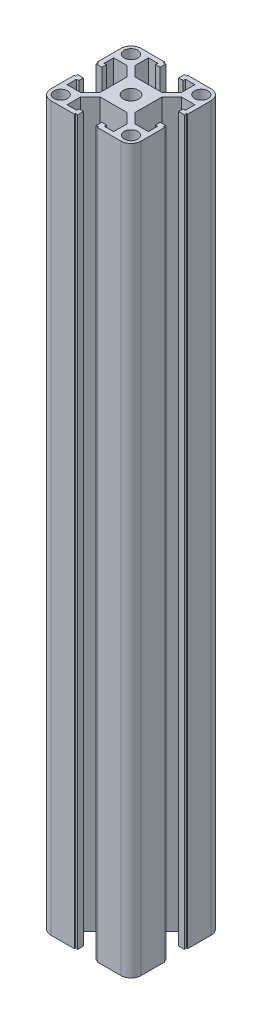
SolidWorks part; units mm, degrees
ref_plane "主视基准图" through (0, 0, 0) normal (0, 0, 1) x (1, 0, 0)
ref_plane "上视基准图" through (0, 0, 0) normal (0, 1, 0) x (1, 0, 0)
ref_plane "右视基准图" through (0, 0, 0) normal (1, 0, 0) x (0, 0, -1)
sketch "草图1" plane through (0, 0, 0) normal (0, 0, 1) x (1, 0, 0)
  line L0 (0, 0) -> (0, 320)
  dimension "D1" = 320
other "结构构件1"
ref_plane "基准面1" through (0, 0, 0) normal (0, 1, 0) x (-1, 0, 0)
sketch "Sketch16" plane through (0, 0, 0) normal (0, 1, 0) x (-1, 0, 0)
  line L0 (-5.1, 20) -> (-5.1, 19.5)
  line L1 (-5.1, 19.5) -> (-4.1, 19.5)
  line L2 (-4.1, 19.5) -> (-4.1, 17)
  line L3 (-6.1, 18) -> (-10.3, 18)
  line L4 (-15.5, -20) -> (-5.1, -20)
  line L5 (-20, -15.5) -> (-20, -5.1)
  line L6 (15.5, 20) -> (5.1, 20)
  line L7 (20, 15.5) -> (20, 5.1)
  line L8 (0, 14.8756) -> (0, 0) construction
  line L9 (0, 0) -> (14.1675, 0) construction
  line L10 (-10.3, 18) -> (-10.3, 12)
  line L11 (-10.3, 12) -> (-6, 7.7)
  line L12 (-6, 7.7) -> (6, 7.7)
  line L13 (10.3, 12) -> (6, 7.7)
  line L14 (10.3, 18) -> (10.3, 12)
  line L15 (6.1, 18) -> (10.3, 18)
  line L16 (4.1, 19.5) -> (4.1, 17)
  line L17 (5.1, 19.5) -> (4.1, 19.5)
  line L18 (5.1, 20) -> (5.1, 19.5)
  line L19 (-5.1, 20) -> (-15.5, 20)
  line L20 (20, 5.1) -> (19.5, 5.1)
  line L21 (0, 0) -> (-15.5563, 15.5563) construction
  line L22 (0, 0) -> (-15.5563, -15.5563) construction
  line L25 (19.5, 5.1) -> (19.5, 4.1)
  line L26 (19.5, 4.1) -> (17, 4.1)
  line L27 (17, 6.1) -> (17, 4.1)
  line L28 (18, 6.1) -> (17, 6.1)
  line L29 (18, 6.1) -> (18, 10.3)
  line L30 (18, 10.3) -> (12, 10.3)
  line L31 (12, 10.3) -> (7.7, 6)
  line L32 (7.7, 6) -> (7.7, -6)
  line L33 (12, -10.3) -> (7.7, -6)
  line L34 (18, -10.3) -> (12, -10.3)
  line L35 (18, -6.1) -> (18, -10.3)
  line L36 (18, -6.1) -> (17, -6.1)
  line L37 (17, -4.1) -> (17, -6.1)
  line L38 (19.5, -4.1) -> (17, -4.1)
  line L39 (19.5, -5.1) -> (19.5, -4.1)
  line L40 (20, -5.1) -> (19.5, -5.1)
  line L41 (5.1, -20) -> (5.1, -19.5)
  line L42 (5.1, -19.5) -> (4.1, -19.5)
  line L43 (4.1, -19.5) -> (4.1, -17)
  line L44 (6.1, -17) -> (4.1, -17)
  line L45 (6.1, -18) -> (6.1, -17)
  line L46 (6.1, -18) -> (10.3, -18)
  line L47 (10.3, -18) -> (10.3, -12)
  line L48 (10.3, -12) -> (6, -7.7)
  line L49 (6, -7.7) -> (-6, -7.7)
  line L50 (-10.3, -12) -> (-6, -7.7)
  line L51 (-10.3, -18) -> (-10.3, -12)
  line L52 (-6.1, -18) -> (-10.3, -18)
  line L53 (-6.1, -18) -> (-6.1, -17)
  line L54 (-4.1, -17) -> (-6.1, -17)
  line L55 (-4.1, -19.5) -> (-4.1, -17)
  line L56 (-5.1, -19.5) -> (-4.1, -19.5)
  line L57 (-5.1, -20) -> (-5.1, -19.5)
  line L58 (-20, -5.1) -> (-19.5, -5.1)
  line L59 (5.1, -20) -> (15.5, -20)
  line L60 (-20, 5.1) -> (-20, 15.5)
  line L61 (-19.5, -5.1) -> (-19.5, -4.1)
  line L62 (-6.1, 18) -> (-6.1, 17)
  line L63 (-6.1, 17) -> (-4.1, 17)
  line L64 (6.1, 18) -> (6.1, 17)
  line L65 (4.1, 17) -> (6.1, 17)
  line L66 (-19.5, -4.1) -> (-17, -4.1)
  line L71 (-17, -6.1) -> (-17, -4.1)
  line L72 (-18, -6.1) -> (-17, -6.1)
  line L73 (-18, -6.1) -> (-18, -10.3)
  line L74 (-18, -10.3) -> (-12, -10.3)
  line L75 (-12, -10.3) -> (-7.7, -6)
  line L76 (-7.7, -6) -> (-7.7, 6)
  line L77 (-12, 10.3) -> (-7.7, 6)
  line L78 (-18, 10.3) -> (-12, 10.3)
  line L79 (-18, 6.1) -> (-18, 10.3)
  line L80 (-18, 6.1) -> (-17, 6.1)
  line L81 (-17, 4.1) -> (-17, 6.1)
  line L82 (-19.5, 4.1) -> (-17, 4.1)
  line L83 (-19.5, 5.1) -> (-19.5, 4.1)
  line L84 (-20, 5.1) -> (-19.5, 5.1)
  line L85 (20, -5.1) -> (20, -15.5)
  circle A0 centre (0, 0) radius 3.4
  arc A1 (-20, 15.5) -> (-15.5, 20) centre (-15.5, 15.5) cw
  arc A2 (20, 15.5) -> (15.5, 20) centre (15.5, 15.5) ccw
  arc A3 (-15.5, -20) -> (-20, -15.5) centre (-15.5, -15.5) cw
  arc A4 (15.5, -20) -> (20, -15.5) centre (15.5, -15.5) ccw
  circle A5 centre (-15.5563, 15.5563) radius 3
  circle A6 centre (15.5563, 15.5563) radius 3
  circle A7 centre (15.5563, -15.5563) radius 3
  circle A8 centre (-15.5563, -15.5563) radius 3
  point P2 (0, 10)
  point P3 (0, 0)
  point P4 (0, 0)
  point P5 (-20, -20)
  point P6 (20, -20)
  point P7 (20, 20)
  point P8 (-20, 20)
  point P36 (-20, 20)
  point P39 (20, 20)
  dimension "D1" = 20.6
  dimension "D2" = 40
  dimension "D3" = 8.2
  dimension "D4" = 10.2
  dimension "D5" = 12.3
  dimension "D6" = 6.8
  dimension "D7" = 4.5
  dimension "D8" = 45
  dimension "D12" = 6
  dimension "D13" = 22
  dimension "D9" = 0.5
  dimension "D10" = 2
  dimension "D11" = 12
  dimension "D16" = 3
  dimension "D17" = 2
